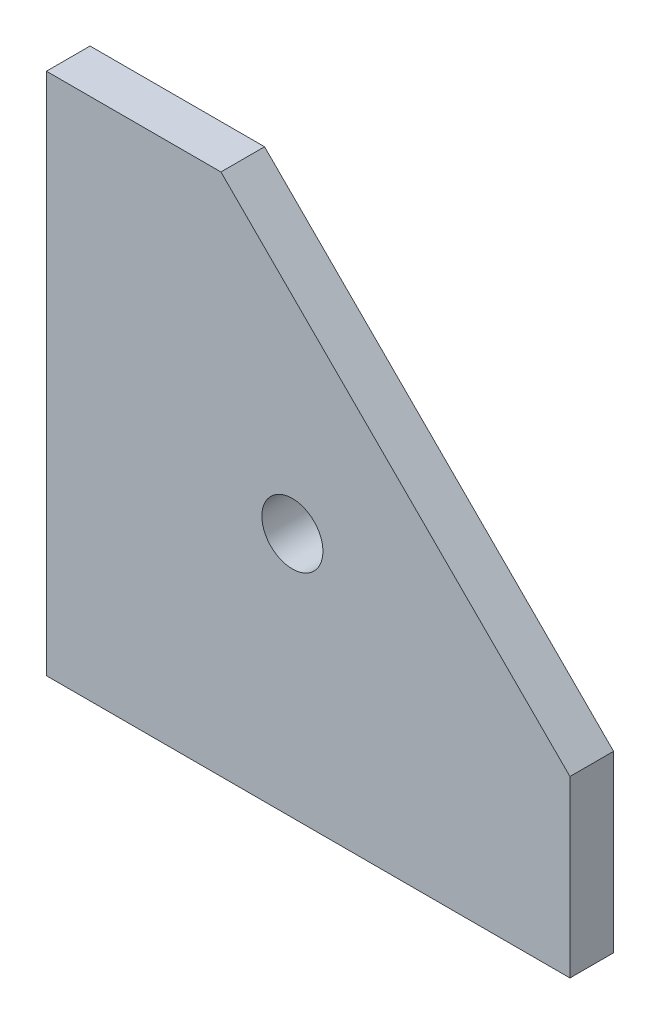
from build123d import *

# Parameters (mm, degrees)
EXTRUDE_1_DEPTH     = 10
HOLE_WIZARD_M16_1_D = 14


with BuildPart() as part:
    # 草图1 → 凸台-拉伸1 (new body)
    with BuildSketch(Plane.XY):
        Polygon((0, 120), (0, 0), (120, 0), (120, 40), (40, 120), align=None)
    extrude(amount=EXTRUDE_1_DEPTH)

    # M16 螺纹孔1 (through all)
    with Locations(Plane(origin=(0, 0, 0), x_dir=(-1, 0, 0), z_dir=(0, 0, -1))):
        with Locations((-56.380361078, 56.380361078)):
            Hole(HOLE_WIZARD_M16_1_D / 2)


solid = part.part
